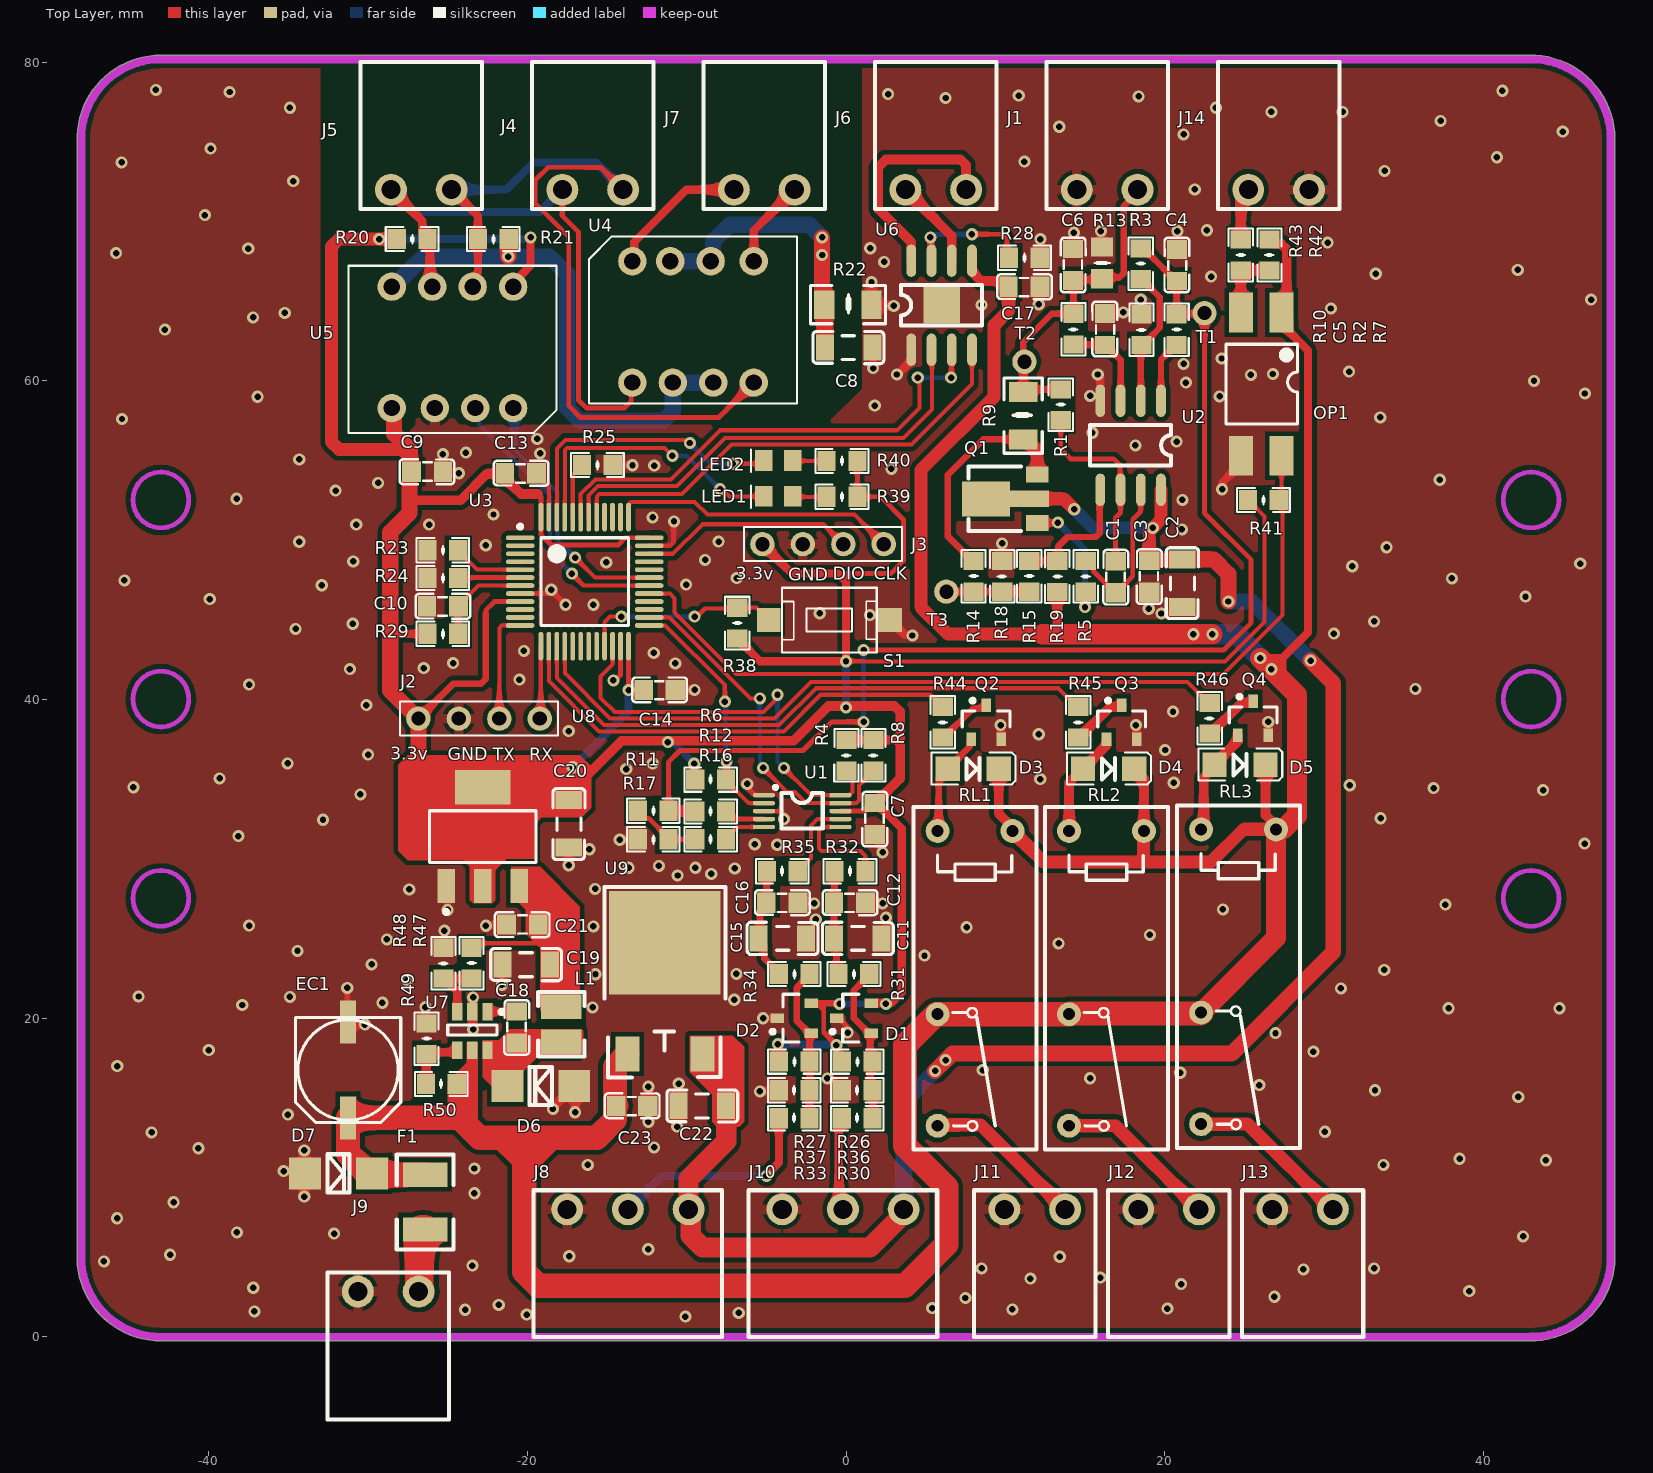
[diagram p0: Top Layer view]
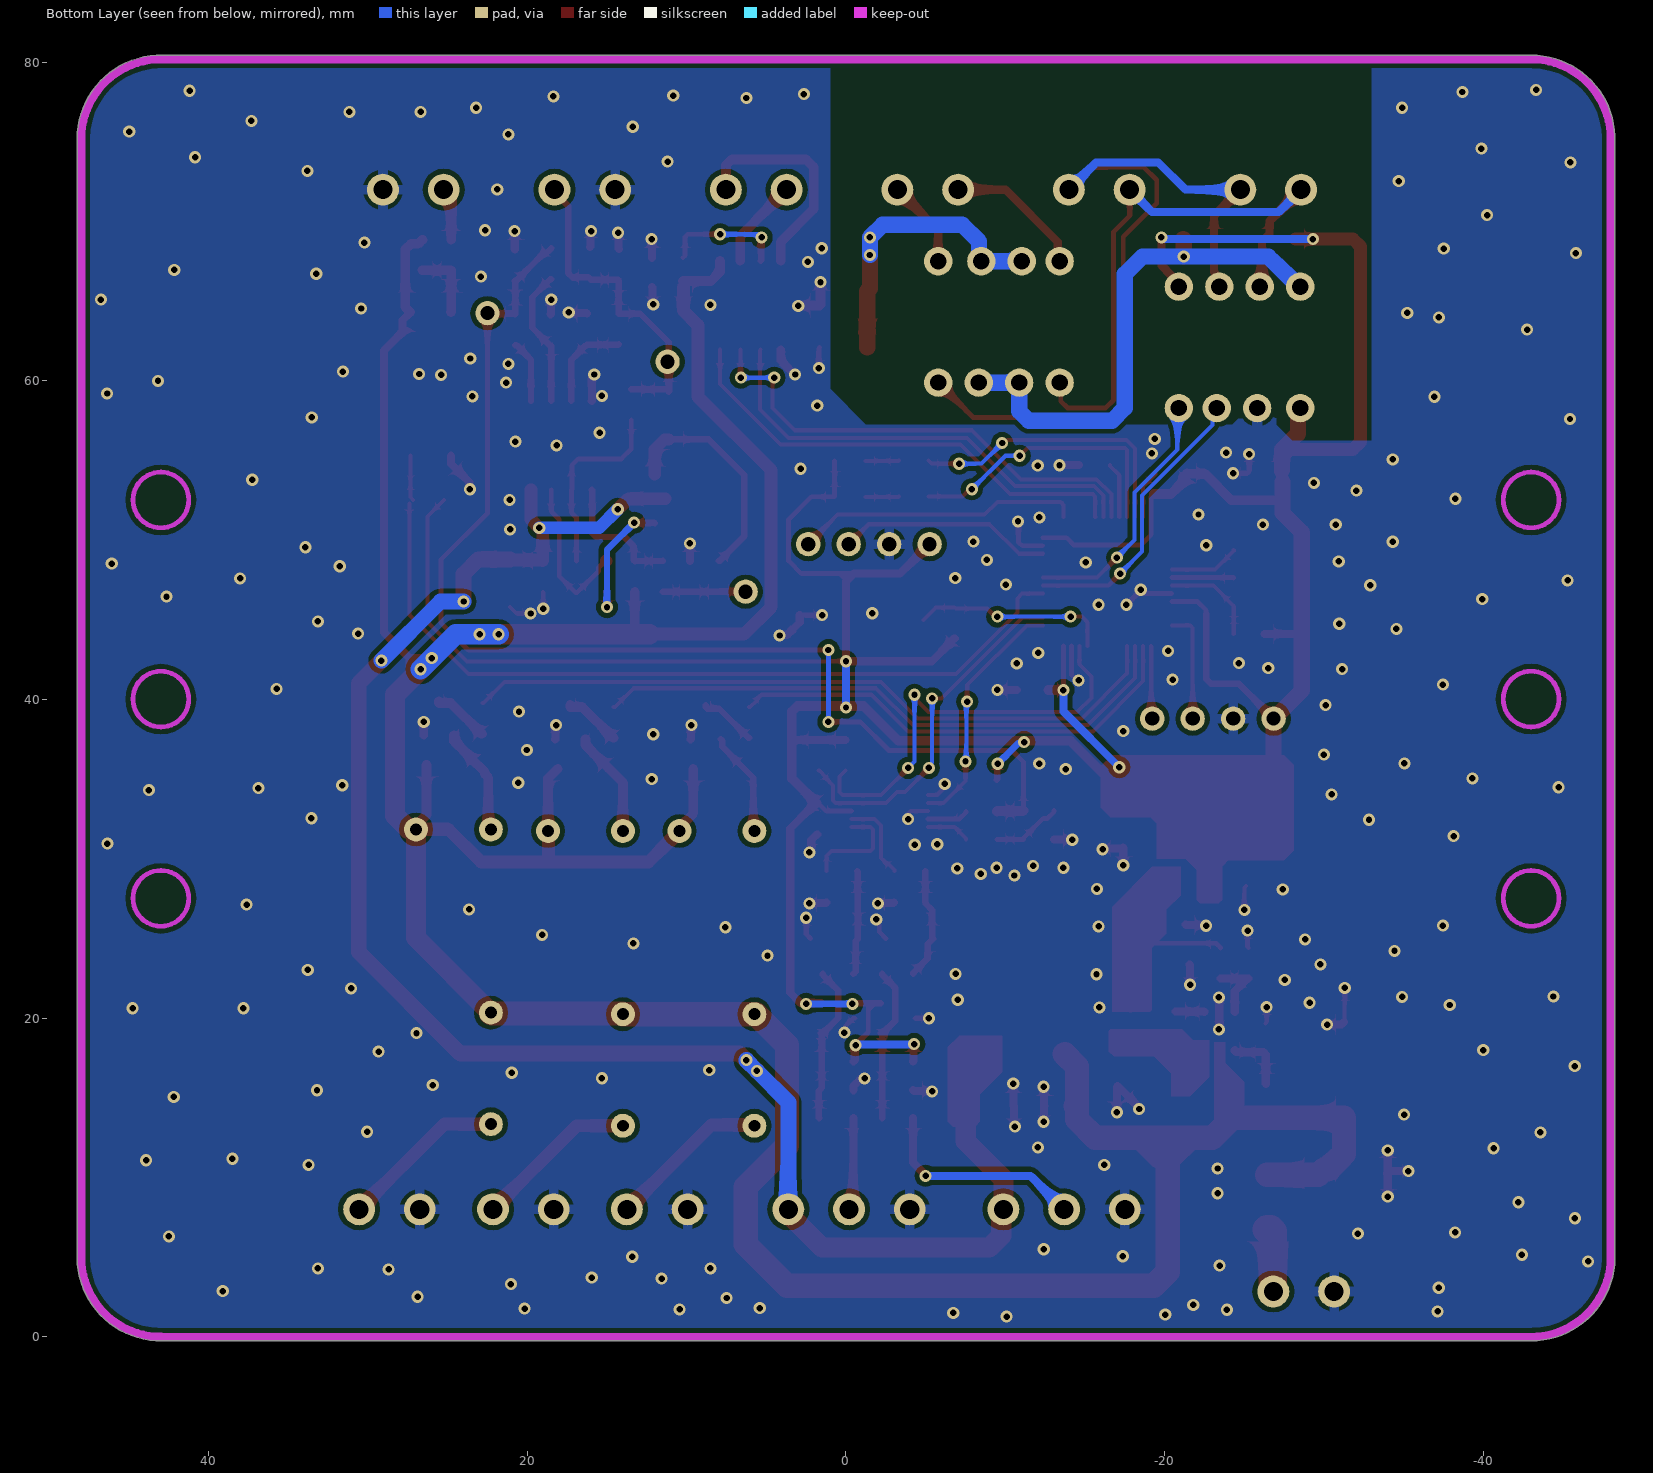
[diagram p1: Bottom Layer view, seen from below]
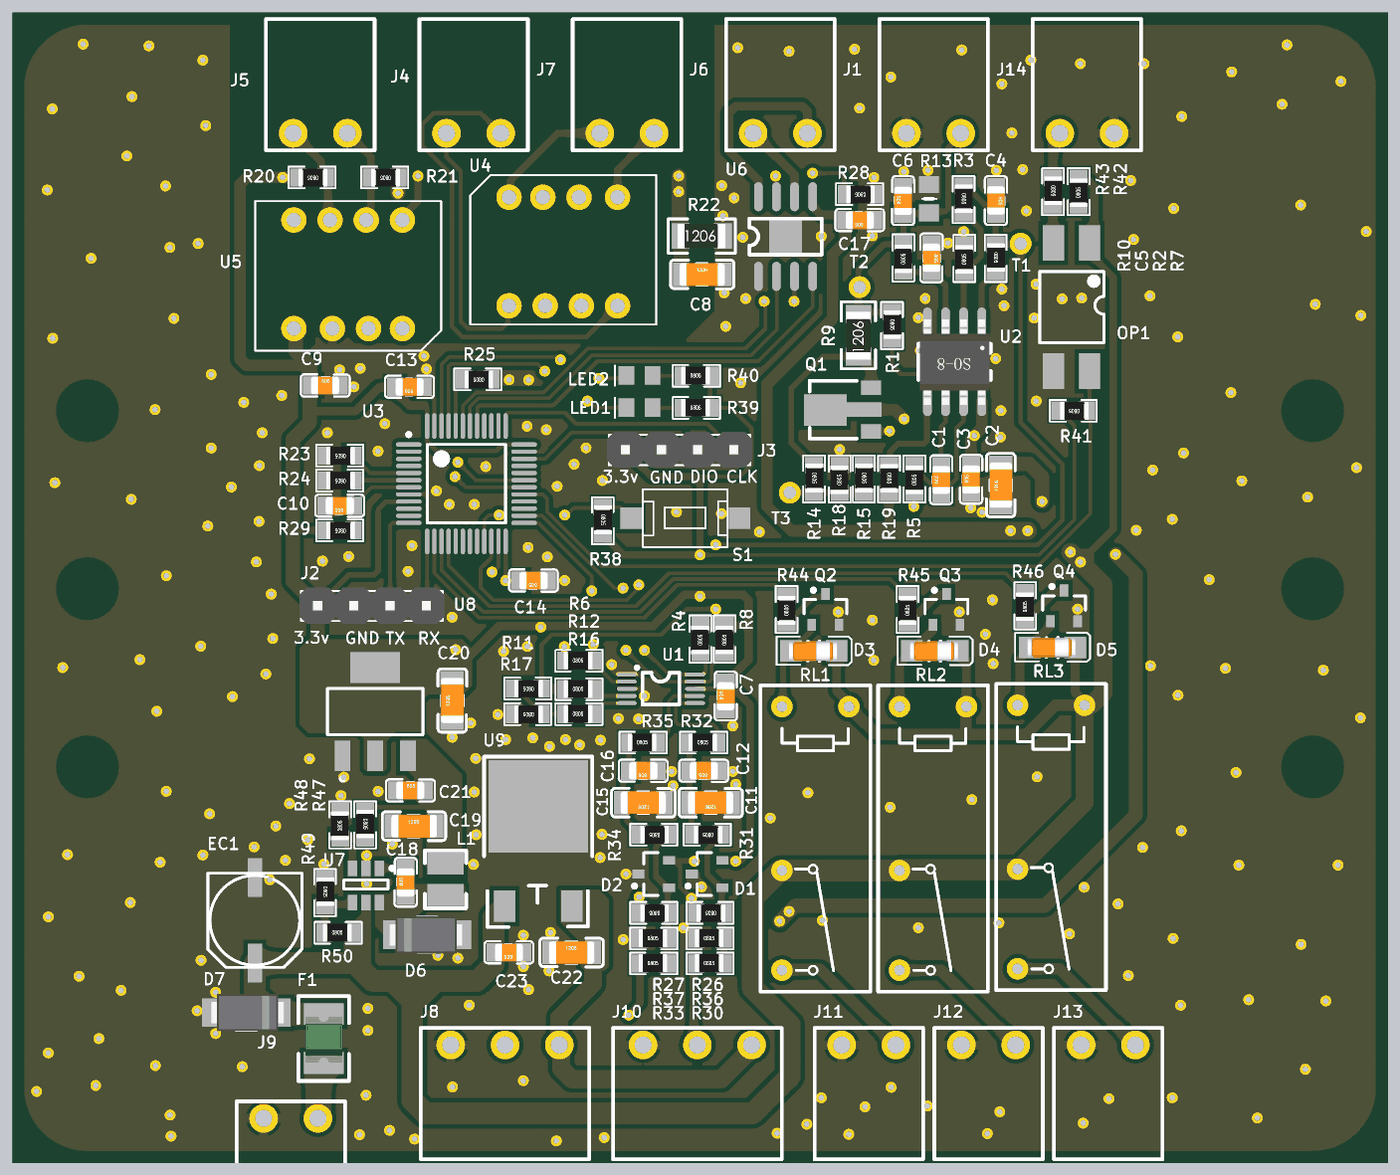
[diagram p2: 3D render of the assembled board from above, using the file's embedded part models]
# Altium PCB MISC82194.PcbDoc (part 1 of 2)
Units mm, origin at the board's own origin, x right, y up, seen from the top; angles counter-clockwise.
Board outline 96.51 x 80.7 mm, 2 copper layers (Top Layer, Bottom Layer); 120 components, 77 nets, 344 pads, 317 vias.
Unrouted connection lines stored in the file: 85.

## Layer stack, top to bottom (the 12.6 mil dielectric is the usual default, probably not edited)
Top Solder: solder mask 0.0102, Solder Resist, Dk 3.5
Top Layer: signal copper 0.0356
Dielectric 1: dielectric 0.32, FR-4, Dk 4.8
Bottom Layer: signal copper 0.0356
Bottom Solder: solder mask 0.0102, Solder Resist, Dk 3.5

## Board outline
-48.235,4.551 cw(c-48,4.648) -48.254,4.648 -48.254,75.336 cw(c-48,75.336) -48.251,75.378 cw(c-43,75.188) -43,80.442 43.205,80.442 cw(c43.205,80.188) 43.28,80.431 cw(c43,75.184) 48.254,75.184 48.254,4.674 cw(c48,4.674) 48.237,4.582 cw(c43,5.004) 43.311,-0.241 cw(c43.231,0) 43.231,-0.254 -43,-0.254 cw(c-43,5)

## Design rules (kind name [scope] priority, off if disabled: settings)
Clearance Clearance_1 [InPolygon] p1: gap=0.508 ignorepadtopadclearanceinfootprint=FALSE except(0: Arc-Hole Track-Hole SMDPad-Hole THPad-Hole Via-Hole Fill-Hole Poly-Hole Region-Hole Text-Hole; 0.3: Arc-Fill Arc-Poly Arc-Region Track-Fill Track-Poly Track-Region SMDPad-Fill SMDPad-Poly SMDPad-Region THPad-Fill THPad-Poly THPad-Region Via-Fill Via-Poly Via-Region Fill-Fill Fill-Poly Fill-Region Poly-Poly Poly-Region Region-Region)
Clearance [All] p2: gap=0.152 ignorepadtopadclearanceinfootprint=FALSE except(0: Arc-Hole Track-Hole SMDPad-Hole THPad-Hole Via-Hole Fill-Hole Poly-Hole Region-Hole Text-Hole; 0.2: Arc-Fill Arc-Poly Arc-Region Track-Fill Track-Poly Track-Region SMDPad-Fill SMDPad-Poly SMDPad-Region THPad-Fill THPad-Poly THPad-Region Via-Fill Via-Poly Via-Region Fill-Fill Fill-Poly Fill-Region Poly-Poly Poly-Region Region-Region)
Height [All] p1: minheight=0 maxheight=254 prefheight=12.7
PlaneConnect [All] p1: planeconnectstyle=Relief reliefexpansion=0.508 reliefentries=4 reliefconductorwidth=0.635 reliefairgap=0.254
PolygonConnect [All] p1: thpad.connectstyle=Relief thpad.reliefconductorwidth=0.635 thpad.reliefentries=4 thpad.polygonreliefangle="90 Angle" thpad.airgapwidth=0.254 smdpad.connectstyle=Direct smdpad.reliefconductorwidth=0.635 smdpad.reliefentries=4 smdpad.polygonreliefangle="90 Angle" smdpad.airgapwidth=0.254 via.connectstyle=Direct via.reliefconductorwidth=0.635 via.reliefentries=4 via.polygonreliefangle="90 Angle" via.airgapwidth=0.254
RoomDefinition 真空计模拟量485合集-PWOER [InComponentClass('真空计模拟量485合集-PWOER')] p1: confinementstyle=ConfineIn formatcopy=TRUE lockcomponents=FALSE outline -243.093,-122.119 -192.293,-122.119 -192.293,-96.719 -243.093,-96.719
RoomDefinition 真空计模拟量485合集-DMCU [InComponentClass('真空计模拟量485合集-DMCU')] p2: confinementstyle=ConfineIn formatcopy=TRUE lockcomponents=FALSE outline -243.093,-122.119 -192.293,-122.119 -192.293,-96.719 -243.093,-96.719
RoutingVias [All] p1: holewidth=0.711 width=1.27 viastyle="Through Hole" minholewidth=0.305 minwidth=0.508 maxholewidth=0.711 maxwidth=1.27
SolderMaskExpansion [All] p1: expansion=0 istentingtop=FALSE
Width [All] p1: maxlimit=2.54 minlimit=0.254 preferedwidth=0.254
28 further rules are at their usual default settings.

## Classes and differential pairs
component class 真空计模拟量485合集-PWOER: C18 C19 C20 C21 C22 C23 D6 D7 EC1 F1 J4 J5 J6 J7 J8 J9 J10 J11 J12 J13 J14 L1 R47 R48 R49 R50 U7 U8 U9
component class 真空计模拟量485合集-DMCU: C1 C2 C3 C4 C5 C6 C7 C8 C9 C10 C11 C12 C13 C14 C15 C16 C17 D1 D2 D3 D4 D5 J1 J2 J3 LED1 LED2 OP1 Q1 Q2 Q3 Q4 R1 R2 R3 R4 R5 R6 R7 R8 R9 R10 R11 R12 R13 R14 R15 R16 R17 R18 R19 R20 R21 R22 R23 R24 R25 R26 R27 R28 R29 R30 R31 R32 R33 R34 R35 R36 R37 R38 R39 R40 R41 R42 R43 R44 R45 R46 RL1 RL2 RL3 S1 T1 T2 T3 U1 U2 U3 U4 U5 U6

## Components (designator, comment, footprint, x,y, rotation, side; value= is the part's Value field where it differs from the comment)
C1 "104" 0805-C-I 16.9,46.7 r90 top
C2 "10uf" 1206-C-I 21.062,45.767 r90 top
C3 "104" 0805-C-I 19,46.735 r90 top
C4 "104" 0805-C-I 20.801,68.25 r270 top
C5 "104" 0805-C-I 16.275,64.231 r270 top
C6 "104" 0805-C-I 14.225,66.296 r90 top
C7 "104" 0805-C-I 1.775,31.519 r90 top
C8 "102-2KV" 1206-C-I -1.383,62.138 r0 top
C9 "104" 0805-C-I -27.281,54.325 r0 top
C10 "104" 0805-C-I -24.319,45.825 r180 top
C11 "NC" 1206-C-I 2.283,24.962 r180 top
C12 "104" 0805-C-I 1.231,27.225 r180 top
C13 "104" 0805-C-I -19.419,54.175 r180 top
C14 "104" 0805-C-I -10.719,40.575 r180 top
C15 "NC" 1206-C-I -2.447,24.962 r180 top
C16 "104" 0805-C-I -3.019,27.225 r180 top
C17 "104" 0805-C-I 12.181,65.875 r180 top
C18 "104" 0805-C-I -20.693,18.444 r90 top
C19 "22uf" 1206-C-I -21.616,23.407 r0 top
C20 "10uf" 1206-C-I -17.438,30.647 r90 top
C21 "104" 0805-C-I -21.3,25.9 r0 top
C22 "22uf" 1206-C-I -10.553,14.538 r0 top
C23 "104" 0805-C-I -12.441,14.47 r180 top
D1 "BTA54S" SOT23_L 0.5,20 r180 top
D2 "BTA54S" SOT23_L -3.25,20 r180 top
D3 "4148" D1206 8.05,35.575 r0 top
D4 "4148" D1206 16.55,35.575 r0 top
D5 "4148" D1206 24.8,35.825 r0 top
D6 "SS34" DO-SMA-I -19,15.75 r0 top
D7 "SS34" DO-SMA-I -32,10.25 r180 top
EC1 "100UF" C6.3X6.3 -31.25,16.75 r90 top
F1 "PPTC" 1210-F -26.518,8.433 r90 top
J1 "Sensor" 3.81-2P-90 16.393,70.806 r180 top
J2 "xh2.54" CON4 -23.03,38.8 r180 top
J3 "xh2.54" CON4 -1.44,49.75 r180 top
J4 "KF2EDG-3.81-2P" 3.81-2P-90 -15.893,70.806 r180 top
J5 "KF2EDG-3.81-2P" 3.81-2P-90 -26.655,70.806 r180 top
J6 "KF2EDG-3.81-2P" 3.81-2P-90 5.631,70.806 r180 top
J7 "KF2EDG-3.81-2P" 3.81-2P-90 -5.131,70.806 r180 top
J8 "KF2EDG-3.81-3P" 3.81-3P-90 -13.69,9.2 r0 top
J9 "KF2EDG-3.81-2P" 3.81-2P-90 -28.727,4.039 r0 top
J10 "KF2EDG-3.81-3P" 3.81-3P-90 -0.19,9.2 r0 top
J11 "KF2EDG-3.81-2P" 3.81-2P-90 11.845,9.194 r0 top
J12 "KF2EDG-3.81-2P" 3.81-2P-90 20.25,9.194 r0 top
J13 "KF2EDG-3.81-2P" 3.81-2P-90 28.655,9.194 r0 top
J14 "KF2EDG-3.81-2P" 3.81-2P-90 27.155,70.806 r180 top
L1 "4.7UH" L-252012 -17.868,19.625 r90 top
LED1 "0805" LED[0805] -4.25,52.75 r0 top
LED2 "0805" LED[0805] -4.25,55 r0 top
OP1 "EL817" EL-817 27.34,64.3 r270 top
Q1 "S8050" SOT-89-3-1 10.4,52.6 r90 top
Q2 "S8050" SOT23_L 8.8,38.575 r90 top
Q3 "S8050" SOT23_L 17.3,38.575 r90 top
Q4 "S8050" SOT23_L 25.55,38.825 r90 top
R1 "4.7k" 0805-R-I 13.5,58.5 r270 top
R2 "10k" 0805-R-I 18.525,63.215 r90 top
R3 "30k" 0805-R-I 18.525,67.347 r270 top
R4 "10k" 0805-R-I 0,36.5 r90 top
R5 "100R" 0805-R-I 15.025,47.735 r90 top
R6 "10k" 0805-R-I -8.5,35 r0 top
R7 "1k" 0805-R-I 20.775,63.215 r270 top
R8 "10k" 0805-R-I 1.7,36.5 r90 top
R9 "100" 1206-R-I 11.1,56.4 r90 top
R10 "1k" 0805-R-I 14.25,63.25 r90 top
R11 "10k" 0805-R-I -12.1,33 r180 top
R12 "0" 0805-R-I -8.5,33 r0 top
R13 "" R[0805] 16.1,67.4 r270 top
R14 "9100" 0805-R-I 8.025,47.735 r270 top
R15 "4.7k" 0805-R-I 11.525,47.735 r270 top
R16 "0" 0805-R-I -8.5,31.25 r0 top
R17 "10k" 0805-R-I -12.1,31.2 r180 top
R18 "1201" 0805-R-I 9.775,47.735 r90 top
R19 "2004/NC" 0805-R-I 13.288,47.722 r270 top
R20 "10k" 0805-R-I -27.235,68.875 r180 top
R21 "10k" 0805-R-I -22.135,68.875 r180 top
R22 "1M" 1206-R-I -1.3,64.8 r0 top
R23 "10k" 0805-R-I -25.3,49.35 r180 top
R24 "10k" 0805-R-I -25.3,47.6 r180 top
R25 "10k" 0805-R-I -15.6,54.7 r180 top
R26 "1M" 0805-R-I 0.7,17.25 r180 top
R27 "1M" 0805-R-I -3.25,17.25 r180 top
R28 "0.15R" 0805-R-I 11.2,67.7 r180 top
R29 "10k" 0805-R-I -25.3,44.1 r180 top
R30 "100k" 0805-R-I 0.7,13.75 r0 top
R31 "1k" 0805-R-I 0.5,22.75 r180 top
R32 "0" 0805-R-I 0.25,29.25 r0 top
R33 "100k" 0805-R-I -3.25,13.75 r0 top
R34 "1k" 0805-R-I -3.25,22.75 r180 top
R35 "0" 0805-R-I -4,29.25 r0 top
R36 "30k" 0805-R-I 0.7,15.5 r0 top
R37 "30k" 0805-R-I -3.25,15.5 r0 top
R38 "10k" 0805-R-I -6.8,44.8 r270 top
R39 "10k" 0805-R-I -0.25,52.75 r0 top
R40 "10k" 0805-R-I -0.25,55 r0 top
R41 "4.7k" 0805-R-I 26.2,52.5 r180 top
R42 "1k" 0805-R-I 26.55,67.9 r90 top
R43 "4.7k" 0805-R-I 24.8,67.9 r270 top
R44 "4.7k" 0805-R-I 6.05,38.575 r90 top
R45 "4.7k" 0805-R-I 14.55,38.575 r90 top
R46 "4.7k" 0805-R-I 22.8,38.825 r90 top
R47 "124K" 0805-R-I -23.483,23.451 r270 top
R48 "20K" 0805-R-I -25.283,23.451 r90 top
R49 "24K" 0805-R-I -26.3,18.7 r270 top
R50 "124k" 0805-R-I -25.4,15.9 r0 top
RL1 "HF-46F" RY-HF46F 7.988,20.097 r180 top
RL2 "HF-46F" RY-HF46F 16.238,20.097 r180 top
RL3 "HF-46F" RY-HF46F 24.525,20.194 r180 top
S1 "SW" KEY-3*6 -1.041,44.983 r180 top
T1 "" TP-TEST 22.5,64.28 r0 top
T2 "" TP-TEST 11.2,61.23 r0 top
T3 "" TP-TEST 6.3,46.8 r0 top
U1 "ADS1115" MSOP-10 -2.75,33 r0 top
U2 "TL1490" SO-8 19.77,58.75 r270 top
U3 "GD32F103C8T6" LQFP48_N -16.4,47.4 r0 top
U4 "ZLG-SP00S12" ZLG-SP00S12 -9.6,63.7 r0 top
U5 "ZLG-RSM485M" ZLG-RSM485M -24.7,62.1 r180 top
U6 "DRV8872" SOP8-9 4.984,62.337 r90 top
U7 "MP2451" SOT23-6 -23.468,19.225 r270 top
U8 "AMS1117-3.3" "SOT-223 - 3" -22.8,31.4 r0 top
U9 "7812" TO-252 -13.723,17.746 r0 top

## Footprints (in the part's own frame and the unit in brackets; to place one, negate y for a bottom-side part, rotate by r counter-clockwise, add the part's x,y. Pads: shape width x height; smd on the part's side, far side on the other; paste and mask are expansions set on the pad)
3.81-2P-90 [mm]
  round 2 hole 1.2: 1(-1.905,-1.194) 2(1.905,-1.194)
  silkscreen extent -3.81,-9.21 3.81,0.01
3.81-3P-90 [mm]
  round 2 hole 1.2: 1(-3.81,-1.2) 2(0,-1.2) 3(3.81,-1.2)
  silkscreen extent -5.92,-9.22 5.92,0
0805-C-I [mil]
  rect 47.24x50 smd: 1(0,-1)
  rect 45x50 smd: 2(78,-1)
  silkscreen extent -29,-32 106,30, body extent -1,-26 77,24, height 30
0805-R-I [mil]
  rect 45x50 smd: 1(-38,-1) 2(38,-1)
  silkscreen extent -65,-31 65,29, body extent -42,-25 37,24, height 19
1206-C-I [mm]
  rect 1.13x1.651 smd: 1(0.053,-0.038) 2(3.033,-0.038)
  silkscreen extent -0.69,-1.06 3.76,0.96, body extent -0.06,-0.85 3.14,0.75, height 1
1206-R-I [mm]
  rect 1.27x1.8 smd: 1(-0.072,-0.017) 2(2.908,-0.017)
  silkscreen extent -0.94,-1.22 3.77,1.18, body extent -0.28,-0.88 3.07,0.85, height 0.85
1210-F [mil]
  rect 60x110 smd: 1(-66.7,-3.9) 2(68.3,-3.9)
  silkscreen extent -117,-74 118,66, body extent -66,-55 61,47, height 27
C6.3X6.3 [mm]
  rect 2.7x1 smd: 1(-3,0) 2(3,0)
  silkscreen extent -3.3,-3.3 3.3,3.3
CON4 [mil]
  round 60 hole 35: 1(-150,0) 2(-50,0) 3(50,0) 4(150,0)
  silkscreen extent -195,-42 196,41, body extent -200,-51 200,49, height 336
D1206 [mil]
  rect 60x60 smd: 1(-65.8,3.2) 2(60.4,3.2)
  silkscreen extent -105,-36 102,43, body extent -72,-25 62,31, height 55
DO-SMA-I [mm]
  rect 2x2 smd: 1(1.948,-0.012) 2(-2.252,-0.012)
  silkscreen extent -0.85,-1.21 0.55,1.19, body extent -2.84,-1.32 2.36,1.28, height 2.53
EL-817 [mm]
  rect 2.5x1.5 smd: 1(0,0) 2(0,-2.54) 3(9,-2.54) 4(9,0)
  silkscreen extent 2,-3.5 7,1
KEY-3*6 [mm]
  rect 1.5x1.5 smd: 1(-3.81,0) 2(3.81,0)
  silkscreen extent -2.97,-2.03 2.97,2.03
L-252012 [mm]
  rect 1.524x2.54 smd: 1(-1.1,0) 2(1.1,0)
  silkscreen extent -2.03,-1.45 2.03,1.45
LED[0805] [mm] "0805"
  rect 1.1x1.3 smd: 1(0.92,0) 2(-0.92,0)
  silkscreen extent -1.72,-0.71 -1.72,0.69
LQFP48_N [mm] "Thin QFP, 48-Leads, Body 7x7mm, Pitch 0.5mm, IPC Medium Density"
  oval 1.8x0.3 smd: 1(-4.05,2.75) 2(-4.05,2.25) 3(-4.05,1.75) 4(-4.05,1.25) 5(-4.05,0.75) 6(-4.05,0.25) 7(-4.05,-0.25) 8(-4.05,-0.75) 9(-4.05,-1.25) 10(-4.05,-1.75) 11(-4.05,-2.25) 12(-4.05,-2.75) 25(4.05,-2.75) 26(4.05,-2.25) 27(4.05,-1.75) 28(4.05,-1.25) 29(4.05,-0.75) 30(4.05,-0.25) 31(4.05,0.25) 32(4.05,0.75) 33(4.05,1.25) 34(4.05,1.75) 35(4.05,2.25) 36(4.05,2.75)
  oval 0.3x1.8 smd: 13(-2.75,-4.05) 14(-2.25,-4.05) 15(-1.75,-4.05) 16(-1.25,-4.05) 17(-0.75,-4.05) 18(-0.25,-4.05) 19(0.25,-4.05) 20(0.75,-4.05) 21(1.25,-4.05) 22(1.75,-4.05) 23(2.25,-4.05) 24(2.75,-4.05) 37(2.75,4.05) 38(2.25,4.05) 39(1.75,4.05) 40(1.25,4.05) 41(0.75,4.05) 42(0.25,4.05) 43(-0.25,4.05) 44(-0.75,4.05) 45(-1.25,4.05) 46(-1.75,4.05) 47(-2.25,4.05) 48(-2.75,4.05)
  silkscreen extent -4.17,-2.75 2.75,3.57, body extent -3.5,-3.5 3.5,3.5, height 1.6
MSOP-10 [mm]
  oval 1.4x0.28 smd mask+0.051: 1(-2.4,1) 2(-2.4,0.5) 3(-2.4,0) 4(-2.4,-0.5) 5(-2.4,-1) 6(2.4,-1) 7(2.4,-0.5) 8(2.4,0) 9(2.4,0.5) 10(2.4,1)
  silkscreen extent -1.75,-1.1 1.29,1.56, body extent -2.2,-1.19 2.42,1.19, height 1.27
R[0805] [mil] "0805"
  rect 47.24x55 smd: 1(-39,-1) 2(39,-1)
  silkscreen extent 0,-20 0,19, body extent -60,-26 62,25, height 51
RY-HF46F [mm]
  round 1.5 hole 0.75: 1(-2.462,-11.653) 2(2.238,-11.653) 3(2.238,-0.153) 4(2.238,6.847)
  silkscreen extent -3.96,-13.15 3.74,8.35
SO-8 [mil]
  oval 80x24 smd: 1(0,0) 2(0,-50) 3(0,-100) 4(0,-150) 5(220,-150) 6(220,-100) 7(220,-50) 8(220,0)
  silkscreen extent 60,-175 160,25, body extent -7,-171 229,21, height 67
SOP8-9 [mil]
  oval 80x24 smd: 1(-15,35) 2(-15,-15) 3(-15,-65) 4(-15,-115) 5(205,-115) 6(205,-65) 7(205,-15) 8(205,35)
  rect 90.55x90.55 smd: 9(95,-40)
  silkscreen extent 45,-140 145,60
SOT23-6 [mm]
  rect 1.1x0.65 smd: 1(-1.175,0.968) 2(-1.175,0.018) 3(-1.175,-0.932) 4(1.225,-0.932) 5(1.225,0.018) 6(1.225,0.968)
  silkscreen extent -1.3,-1.53 0.28,1.97, body extent -1.16,-1.4 1.18,1.44, height 1
SOT23_L [mm] "SOT23, 3-Leads, Body 2.9x1.3mm, Pitch 0.95mm, Lead Span 2.3mm - Reverse Pinning, IPC High Density"
  rect 0.85x0.6 smd: 1(1.075,0) 2(-1.075,-0.95) 3(-1.075,0.95)
  silkscreen extent -0.3,-1.5 1.47,1.5, body extent -0.7,-1.5 0.7,1.5, height 1.1
SOT-89-3-1 [mil]
  rect 40x55 smd: 1(-60,-63.28) 2(60,-63.28)
  rect 86.61x118.11 smd: 3(-0.94,63.28)
  rect 40x110.24 smd: 3(0,-37.11)
  silkscreen extent -80,-23 80,107
"SOT-223 - 3" [mm]
  rect 1.1x2.15 smd: 1(-2.3,-3.1) 2(0,-3.1) 3(2.3,-3.1)
  rect 3.5x2.15 smd: 2(0,3.1)
  silkscreen extent -3.35,-4.85 3.35,1.63
TO-252 [mm]
  rect 1.5x2.2 smd: 1(0,0) 3(4.723,0.004)
  rect 7x6.5 smd: 2(2.361,7)
  silkscreen extent -1.44,-1.46 6.16,10.5
TP-TEST [mil]
  round 60 hole 35: 1(0,-1.2)
ZLG-RSM485M [mil]
  round 70 hole 40: 1(-150,150) 2(-56.41,150) 3(43.59,150) 4(150,150) 5(150,-150) 6(50,-150) 7(-50,-150) 8(-150,-150)
  silkscreen extent -257,-202 257,211
ZLG-SP00S12 [mil]
  round 70 hole 40: 1(-150,150) 2(-56.41,150) 3(43.59,150) 4(150,150) 5(150,-150) 6(50,-150) 7(-50,-150) 8(-150,-150)
  silkscreen extent -257,-202 257,211

## Part data
C1 C2 C3 C4 C5 C6 C7 C8 C9 C10 C11 C12 C13 C14 C15 C16 C17 C18 C19 C20 C21 C22 C23: library part Cap
D1 D2: library part DODI-II
D3 D4 D5: library part DIODE
D6 D7: library part DIODE-SBD
EC1: library part "Cap Pol"
F1: library part FUSE-PTC
J1 J4 J5 J6 J7 J9 J11 J12 J13 J14: library part CON2
J2 J3: library part CON4
J8 J10: library part CON3
L1: library part INDUCTOR
LED1 LED2: library part LED
OP1: library part Optocoupler
Q1 Q2 Q3 Q4: library part BJT-NPN
R1 R2 R3 R4 R5 R6 R7 R8 R9 R10 R11 R12 R14 R15 R16 R17 R18 R19 R20 R21 R22 R23 R24 R25 R26 R27 R29 R30 R31 R32 R33 R34 R35 R36 R37 R38 R39 R40 R41 R42 R43 R44 R45 R46 R47 R48 R49 R50: library part R1
R13 R28: library part R
RL1 RL2 RL3: library part RELAY4
S1: library part Button
T1 T2 T3: library part TP-TEST1
U2: library part OPAPM-2
U3: library part STM32F103C8T6, "STM32 ARM-based 32-bit MCU with 64 Kbytes Flash, 48-pin LQFP, Industrial Temperature"
U7: library part LT1933
U8: library part AMS1117
U9: library part LM7805

## Via types
v1: diameter 0.762, hole 0.406, Top Layer to Bottom Layer, 317 vias

## Nets (pads, with @x,y where several pads share a name; then routed paths per layer and width w, separated by ;. In a path a pad name is that pad's centre, name@x,y a point inside that pad or via, vN(x,y) a via of type N, cw(c..) or ccw(c..) an arc to the next point about the centre after c; other vN are vias at no path point)
3.3V: C7.2 C9.1 C13.2 C14.2 C20.2 D1.2 D2.2 J2.4 J3.4 R4.2 R6.1 R8.2 R20.2 R26.2 R27.2 R29.2 R38.2 R39.2 R40.2 R41.2 U1.8 U3.9 U3.24 U3.36 U3.48 U5.4 U5.8 U8.2 | length 242.5
  Top Layer w0.254: v1(0,42.4) 23.8,42.4 26.264,44.864 26.264,51.497 R41.2@25.235,52.525
  Top Layer w0.305: -22.6,45.4 -22.6,45.6 -22.05,46.15 U3.9@-20.45,46.15 ; -19.329,52.9 -19.15,52.721 U3.48@-19.15,51.45 -19.148,51.448 -19.148,50.348 -18.5,49.7 -14.3,49.7 -13.85,50.15 U3.36@-12.35,50.15 ; v1(-13.65,40.594) U3.24@-13.65,43.35 ; -1.712,20.925 -1.712,20.812 -1.4,20.5 ; -1.4,20.925 -1.4,20.5 ; v1(-0.6,18.3) -1.4,19.1 -1.4,20.5 ; U1.8@-0.35,33 1.237,33 C7.2@1.736,33.5 ; -0.25,47.65 0,47.65 0.15,47.65 0.4,47.9 ; -0.25,47.9 0.4,47.9 ; R40.2@0.715,54.975 R39.2@0.715,52.725 2.175,52.725 3.6,51.3 3.6,48.7 2.8,47.9 0.4,47.9
  Top Layer w0.406: J2.4@-26.84,38.8 -24.64,41 -22.9,41 -22.6,41.3 -22.6,45.4 ; v1(-9.525,35.966) -9.495,35.936 -9.495,35.004 R6.1@-9.465,34.975 ; D2.2@-2.175,20.95 -2.15,20.925 -1.712,20.925 -1.4,20.925 -0.425,20.925 v1(-0.4,20.9)
  Top Layer w0.508: -28.6,44 -28.475,44.125 R29.2@-26.265,44.125 ; U5.8@-20.89,65.91 -20.89,66.162 -19.8,67.252 v1(-19.8,69) ; -17.4,34.3 -17.4,35.115 -17.199,35.316 -17.199,35.701 v1(-17.15,35.75) ; R38.2@-6.825,43.835 -6.762,43.835 -6.444,43.517 -6.444,43.454 -5.391,42.4 v1(0,42.4) 0,47.4 -0.25,47.65 -0.5,47.9 -3.4,47.9 J3.4@-5.25,49.75 ; v1(-4.279,18.379) -4.247,18.347 -4.247,17.307 R27.2@-4.215,17.275 ; v1(-0.6,18.3) -0.551,18.251 -0.551,17.362 R26.2@-0.465,17.275 ; R4.2@0.025,37.465 R8.2@1.725,37.465 3.102,37.465 3.4,37.168 ; D1.2@1.575,20.95 2.85,20.95 3.5,21.6 3.5,31.9 2.218,33.182 2.117,33.182 C7.2@1.8,33.5 ; C7.2@1.863,33.5 C7.2@2.082,33.718
  Top Layer w0.61: -27.4,52.5 -24.2,52.5 -22.529,54.171 -21.429,54.171 C13.2@-21.4,54.2 -21.133,53.933 -21.133,53.633 -20.4,52.9 -19.329,52.9 ; -17.4,34.3 -17.2,34.3 -14.09,37.41 -3.29,37.41 -1.1,39.6 3.043,39.6 3.4,39.243 3.4,37.168 3.4,35.037 C7.2@2.082,33.718 ; v1(-13.65,40.594) -13.647,40.597 -12.703,40.597 C14.2@-12.7,40.6
  Top Layer w0.813: R20.2@-28.2,68.9 v1(-29.3,68.9) -31.824,68.9 -32.3,68.424 -32.3,56.176 -31.824,55.7 -27.9,55.7 -27.281,55.081 ; C9.1@-27.373,54.392 C9.1@-27.281,54.3
  Top Layer w1.016: U5.4@-28.51,58.29 -28.364,58.144 -28.364,56.683 -27.373,55.692 C9.1@-27.373,54.392 ; -27.4,53.665 -27.4,52.5 -27.4,51.7 -28.6,50.5 -28.6,44 -28.6,40.56 J2.4@-26.84,38.8 -26.84,35.26 -27,35.1
  Bottom Layer w0.406: v1(-11.176,37.333) -11.108,37.265 -10.824,37.265 v1(-9.525,35.966) ; v1(-0.4,20.9) v1(2.5,20.9)
  Bottom Layer w0.508: v1(-29.3,68.9) -19.969,68.9 -19.869,69 v1(-19.8,69) ; v1(-17.15,35.75) -13.65,39.25 v1(-13.65,40.594) ; v1(-4.279,18.379) -4.239,18.339 -0.639,18.339 v1(-0.6,18.3) ; v1(0,39.5) v1(0,42.4)
5.7V: C19.2 C21.2 L1.2 R47.1 U8.3 | length 10
  Top Layer w0.305: R47.1@-23.508,24.416 -23.224,24.7 -18.6,24.7 -18.226,24.326 -18.226,23.098 C19.2@-18.399,22.925
  Top Layer w0.762: C19.2@-18.583,23.37 -18.583,23.109 -18.399,22.925 -18.314,22.925 -17.868,22.479 L1.2@-17.868,20.725
12V: C2.2 C3.2 C22.2 J8.3 J10.3 Q1.3 U2.8 U9.3 | length 108.7
  Top Layer w0.8: Q1.3@11.343,52.6 13.669,52.6 v1(14.326,51.943) ; U2.8@19.77,53.162 19.77,51.291 v1(19.253,50.775) 19.025,50.547 C3.2@19.025,48.716 19.067,48.758 21.058,48.758 C2.2@21.1,48.8
  Top Layer w1: v1(5.588,16.688) 6.68,17.78 24.206,17.78 30.582,24.155 30.582,41.021 v1(29.159,42.443) ; C2.2@21.1,48.8 23.082,48.8 24.003,47.879 v1(24.003,46.152)
  Top Layer w1.27: C22.2@-7.52,14.5 -7.52,12.28 -9.88,9.92 J8.3@-9.88,8 -9.74,7.86 -9.74,6.344 -8.996,5.6 1.5,5.6 3.48,7.58 3.48,7.86 J10.3@3.62,8
  Bottom Layer w0.8: v1(14.326,51.943) 15.494,50.775 v1(19.253,50.775)
  Bottom Layer w1: J10.3@3.62,8 3.62,14.72 v1(5.588,16.688) 6.248,17.348 v1(6.248,17.374) ; v1(24.003,46.152) 25.451,46.152 v1(29.159,42.443)
24V: C17.2 C23.2 D3.2 D4.2 D5.2 D7.2 EC1.1 F1.2 OP1.1 R19.2 R42.2 R50.2 RL1.1 RL1.3 RL2.1 RL2.3 RL3.1 RL3.3 U6.5 U7.5 U9.1 | length 247.9
  Top Layer w0.508: v1(26,42.6) 27.4,42.6 ; v1(26.7,41.9) 27.4,42.6 ; 27.29,41.31 27.4,41.421 27.4,42.6 ; OP1.1@27.34,64.3 27.836,63.804 27.836,63.064 29,61.9 29,44.2 27.4,42.6
  Top Layer w0.61: U6.5@7.905,67.544 7.905,66.833 8.469,66.269 C17.2@10.225,66.269 ; D3.2@9.584,35.656 9.584,32.857 10.45,31.991 RL1.1@10.45,31.75 ; R19.2@13.263,46.757 13.263,44.457 13.62,44.1 ; D4.2@18.084,35.656 18.7,35.04 RL2.1@18.7,31.75 ; v1(21.8,44.1) 21.829,44.129 v1@22.029,44.129 ; D5.2@26.334,35.906 26.334,32.741 26.988,32.088 RL3.1@26.988,31.847 ; R42.2@26.575,68.865 26.842,68.598 27.311,68.598 27.668,68.241 27.668,64.628 OP1.1@27.34,64.3
  Top Layer w0.813: C17.2@10.2,65.9 10.2,64.4 9.3,63.5 9.3,59 4.7,54.4 4.7,45.8 6.4,44.1 12.3,44.1 ; RL1.1@10.45,31.75 12.4,29.8 18.67,29.8 ; RL2.1@18.7,31.75 18.67,31.72 18.67,29.8 ; RL3.1@26.988,31.847 24.947,31.847 22.9,29.8 18.67,29.8
  Top Layer w1.27: 12.3,44.1 13.62,44.1 v1(21.8,44.1) v1(23,44.1) ; RL3.3@22.288,20.347 26.988,25.047 RL3.1@26.988,31.847 27.032,31.891 27.485,31.891 28.3,32.706 28.3,40.3 27.29,41.31 v1(26.7,41.9) v1(26,42.6)
  Top Layer w1.524: F1.2@-26.419,10.168 -29.653,10.168 -29.986,10.5 -30.25,10.5 -31.25,11.5 EC1.1@-31.25,13.75 -24.25,13.75 -23,12.5 -21.6,12.5 ; C23.2@-14.5,14.496 -14.5,13.643 -15.643,12.5 -18.5,12.5 ; C23.2@-14.423,14.496 -14.5,14.573 -14.5,16.968 U9.1@-13.723,17.746 ; RL3.3@22.288,20.347 22.239,20.298 14.048,20.298 RL2.3@14,20.25 RL1.3@5.75,20.25 5.65,20.25 3.7,18.3 3.7,12 6.3,9.4 6.3,5.8 3.7,3.2 -19.307,3.2 -20.2,4.093 -20.2,11.3 ; -21.6,12.5 -20.2,12.5 ; -21.6,12.5 -20.4,11.3 -20.2,11.3 ; -20.2,11.3 -19.7,11.3 -18.5,12.5 ; -20.2,11.3 -20.2,12.5 ; -20.2,12.5 -18.5,12.5
  Bottom Layer w1.27: v1(21.8,44.1) v1(23,44.1) 24.5,44.1 v1(26,42.6) v1(26.7,41.9)
AD-RDY: R6.2 U1.2 U3.25 | length 15.3
  Top Layer w0.254: U3.25@-12.35,44.65 -11.35,44.65 -7.6,40.9 v1(-7.6,39.873) ; v1(-7.5,36.114) -7.5,34.876 -6.124,33.5 U1.2@-5.15,33.5
  Bottom Layer w0.254: v1(-7.6,39.873) -7.55,39.823 -7.55,36.164 v1(-7.5,36.114)
AD-SCL: R4.1 U1.10 U3.22 | length 26.9
  Top Layer w0.254: -15.251,41.6 -15.4,41.451 -15.4,40.1 -14.513,39.213 -5.187,39.213 -4.704,39.696 -4.485,39.915 -4.485,39.978 -4.3,40.163 v1(-4.3,40.3) ; -15.25,41.6 -14.65,42.2 U3.22@-14.65,43.35 ; v1(-3.9,35.705) -2.195,34 0.203,34 0.4,34.197 0.4,35.16 R4.1@0.025,35.535
  Bottom Layer w0.254: v1(-4.3,40.3) -4.3,36.107 -3.9,35.707 v1(-3.9,35.705)
AD-SDA: R8.1 U1.9 U3.26 | length 22.8
  Top Layer w0.254: U3.26@-12.35,45.15 -11.071,45.15 -5.989,40.068 v1(-5.406,40.068) ; v1(-5.2,35.705) -3.695,34.2 -3.2,34.2 -2.5,33.5 U1.9@-0.35,33.5 0.658,33.5 0.806,33.649 0.806,34.616 1.217,35.027 1.217,35.09 1.662,35.535 R8.1@1.725,35.535
  Bottom Layer w0.254: v1(-5.406,40.068) -5.406,36.048 -5.2,35.842 v1(-5.2,35.705)
ADS-AD1: R11.2 R16.1 R17.1 | length 4.4
  Top Layer w0.305: R11.2@-13.065,33.025 -13.065,32.962 -12.646,32.543 -12.389,32.543 -11.135,31.289 R17.1@-11.135,31.225 ; R17.1@-11.135,31.225 R16.1@-9.465,31.225
ADS-AD2: C4.2 R3.1 R7.1 R11.1 R12.1 T1.1 | length 75.2
  Top Layer w0.305: R11.1@-11.135,33.025 -11.135,36.084 -10.419,36.8 -2.7,36.8 -0.9,38.6 v1(1.1,38.6) ; v1(1.1,43.108) 23.708,43.108 25.425,44.825 25.425,48.768 22.5,51.693 T1.1@22.5,64.25
  Top Layer w0.406: R3.1@18.5,68.312 18.868,67.944 19.037,67.944 20.712,66.269 C4.2@20.775,66.269 20.75,66.243 R7.1@20.75,64.18 20.785,64.215 22.465,64.215 T1.1@22.5,64.25
  Top Layer w0.635: R11.1@-11.135,33.025 -11.109,33 -9.491,33 R12.1@-9.465,32.975
  Bottom Layer w0.305: v1(1.1,38.6) v1(1.1,43.108)
ADS-AD3: R35.2 U1.7 | length 5.3
  Top Layer w0.254: R35.2@-3.035,29.225 -3.035,29.288 -2.59,29.733 -2.527,29.733 -2.2,30.059 -2.2,32.1 -1.8,32.5 U1.7@-0.35,32.5
ADS-AD4: R32.2 U1.6 | length 6.7
  Top Layer w0.254: U1.6@-0.35,32 -1.551,32 -1.7,31.851 -1.7,30.649 -1.551,30.5 0.9,30.5 1.215,30.185 R32.2@1.215,29.225
Analog-VIN1: J8.2 R33.1 | length 13.5
  Top Layer w0.508: v1(-5,10.1) -5,10.147 -4.215,10.932 R33.1@-4.215,13.725
  Bottom Layer w0.508: J8.2@-13.69,8 -11.59,10.1 v1(-5,10.1)
Analog-VIN2: J10.2 R30.1 | length 5.8
  Top Layer w0.508: R30.1@-0.465,13.725 -0.465,8.275 J10.2@-0.19,8
CLK: J3.1 U3.37 | length 18
  Top Layer w0.254: U3.37@-13.65,51.45 -13.65,52.212 -13.627,52.235 -13.627,52.251 -13.478,52.4 -9.5,52.4 -8.7,51.6 0.52,51.6 J3.1@2.37,49.75
DIO: J3.2 U3.34 | length 13.5
  Top Layer w0.254: U3.34@-12.35,49.15 -10.845,49.15 -8.995,51 -1.42,51 J3.2@-0.17,49.75
DRV-FAU1: U3.41 U6.4 | length 29.9
  Top Layer w0.254: U3.41@-15.65,51.45 -15.641,51.459 -15.641,52.751 -15.492,52.9 -10.3,52.9 -7.2,56 4.1,56 7.905,59.805 U6.4@7.905,61.956